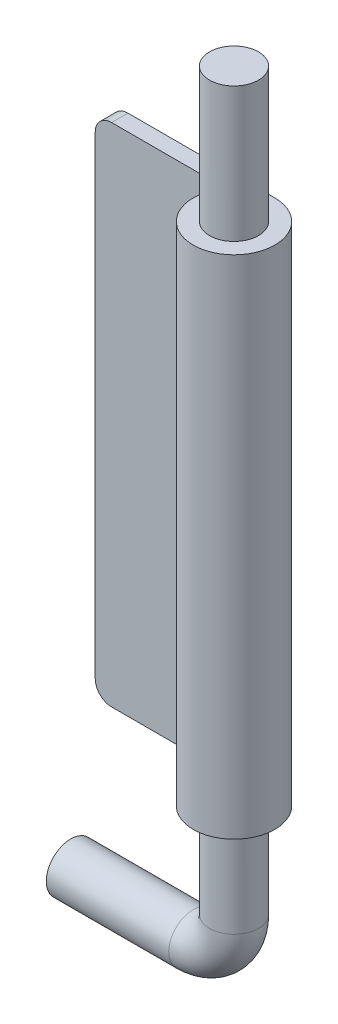
SolidWorks part; units mm, degrees
material "Q235A"
ref_plane "Front Plane" through (0, 0, 0) normal (0, 0, 1) x (1, 0, 0)
ref_plane "Top Plane" through (0, 0, 0) normal (0, 1, 0) x (1, 0, 0)
ref_plane "Right Plane" through (0, 0, 0) normal (1, 0, 0) x (0, 0, -1)
sketch "Sketch1" plane through (0, 0, 0) normal (0, 1, 0) x (1, 0, 0)
  line L0 (0, 5) -> (-20, 5)
  line L1 (0, 3) -> (-20, 3)
  line L2 (-20, 3) -> (-20, 5)
  line L3 (0, 0) -> (-10.9314, 0) construction
  line L4 (-4.8296, 1.2941) -> (-2.8978, 0.7765)
  arc A0 (-4.8296, 1.2941) -> (0, 5) centre (0, 0) ccw
  arc A1 (-2.8978, 0.7765) -> (0, 3) centre (0, 0) ccw
  circle A3 centre (0, 0) radius 5 construction
  circle A4 centre (0, 0) radius 3 construction
  point P9 (4.7815, 1.4619)
  point P14 (3, 0)
  dimension "D1" = 10
  dimension "D3" = 20
  dimension "D4" = 15
  dimension "D2" = 2
extrude "Boss-Extrude1" add sketch "Sketch1" along normal blind 62
sketch "Sketch2" plane through (0, 0, 0) normal (0, 0, 1) x (1, 0, 0)
  line L0 (0, 0) -> (0, 78.5)
  line L1 (0, 0) -> (0, -11.5)
  line L2 (-5, -16.5) -> (-20, -16.5)
  line L3 (5, 62) -> (-5, 62) construction
  arc A0 (0, -11.5) -> (-5, -16.5) centre (-5, -11.5) cw
  point P8 (0, 74.5)
  point P11 (0, -16.5)
  dimension "D3" = 5
  dimension "D4" = 95
  dimension "D1" = 20
  dimension "D2" = 16.5
sweep "Sweep1" add path "Sketch2" circular profile diameter 6 parameters "D3"=6
fillet "Fillet3" radius 2 2 edges at (-20, 0, -4) (-20, 62, -4)
